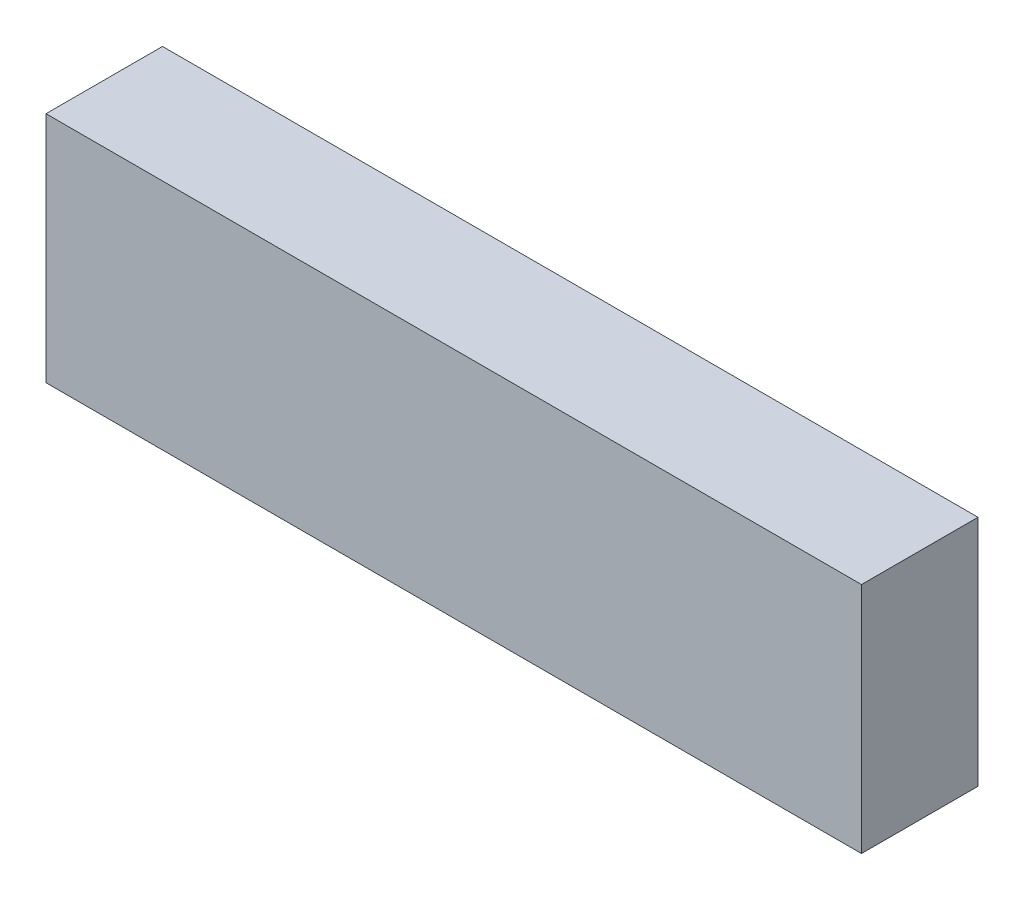
SolidWorks part; units mm, degrees
ref_plane "前视基准面" through (0, 0, 0) normal (0, 0, 1) x (1, 0, 0)
ref_plane "上视基准面" through (0, 0, 0) normal (0, 1, 0) x (1, 0, 0)
ref_plane "右视基准面" through (0, 0, 0) normal (1, 0, 0) x (0, 0, -1)
sketch "草图1" plane through (0, 0, 0) normal (0, 0, 1) x (1, 0, 0)
  line L1 (-35, 10) -> (35, 10)
  line L2 (-35, 10) -> (-35, -10)
  line L3 (-35, -10) -> (35, -10)
  line L4 (35, 10) -> (35, -10)
  line L5 (-35, 10) -> (35, -10) construction
  line L6 (-35, -10) -> (35, 10) construction
  point P0 (0, 0)
  dimension "D1" = 70
  dimension "D2" = 20
extrude "凸台-拉伸1" add sketch "草图1" against normal blind 10
